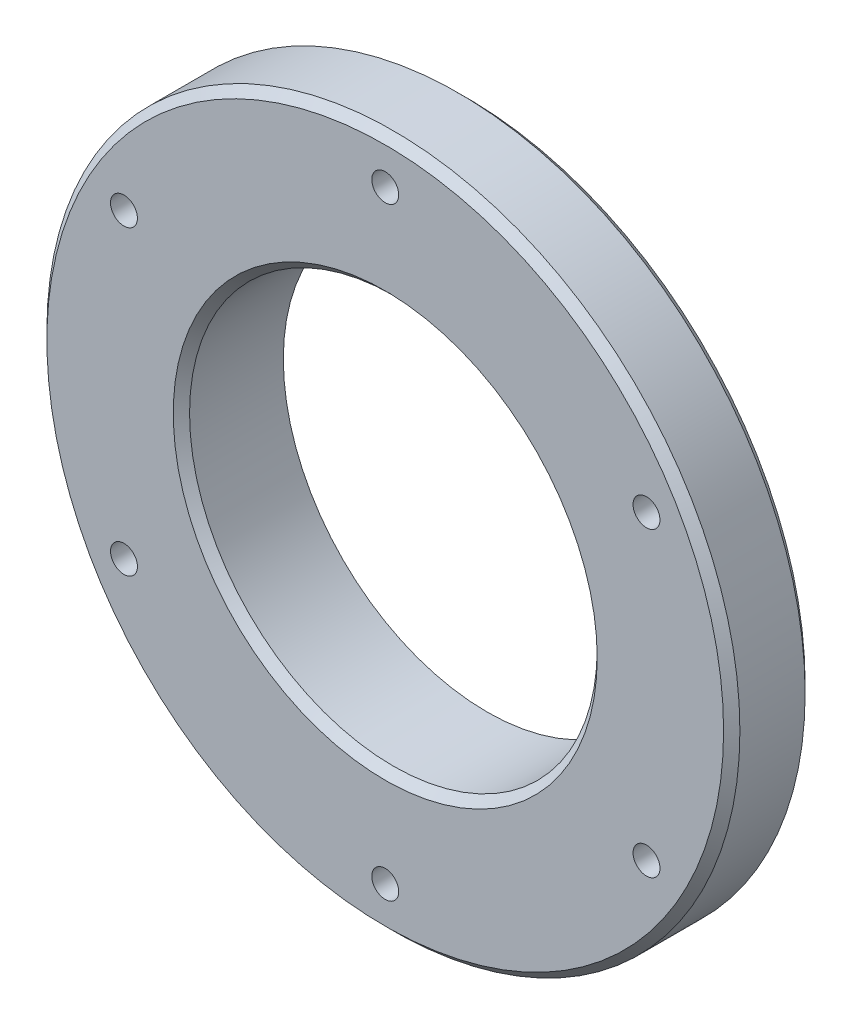
SolidWorks part; units mm, degrees
ref_plane "Front Plane" through (0, 0, 0) normal (0, 0, 1) x (1, 0, 0)
ref_plane "Top Plane" through (0, 0, 0) normal (0, 1, 0) x (1, 0, 0)
ref_plane "Right Plane" through (0, 0, 0) normal (1, 0, 0) x (0, 0, -1)
sketch "Sketch1" plane through (0, 0, 0) normal (0, 0, 1) x (1, 0, 0)
  circle A0 centre (0, 0) radius 42.5
  circle A1 centre (0, 0) radius 25
extrude "Boss-Extrude1" add sketch "Sketch1" along normal blind 10
chamfer "Chamfer1" distance 1 angle 45 3 edges at (42.5, 0, 0) (42.5, 0, 10) (25, 0, 10)
sketch "Sketch2" plane through (0, 0, 10) normal (0, 0, 1) x (1, 0, 0)
  circle A0 centre (0, 37) radius 3.5
  circle A3 centre (32.0434, 18.5009) radius 3.5
  circle A5 centre (32.0444, -18.4991) radius 3.5
  circle A7 centre (0.002, -37) radius 3.5
  circle A9 centre (-32.0414, -18.5009) radius 3.5
  circle A11 centre (-32.0424, 18.4991) radius 3.5
  point P29 (0.001, 0)
  dimension "D1" = 6
hole_wizard "M4x0.7 Tapped Hole1" positions "3DSketch1" profile "Sketch3" tap size "M4x0.7" standard "Ansi Metric"
sketch3d "3DSketch1"
  point P0 (0, 37, 10)
  point P3 (32.0434, 18.5009, 10)
  point P6 (32.0444, -18.4991, 10)
  point P9 (0.002, -37, 10)
  point P12 (-32.0414, -18.5009, 10)
  point P15 (-32.0424, 18.4991, 10)
sketch "Sketch3" plane through (0, 37, 10) normal (1, 0, 0) x (0, -1, 0)
  line L0 (0, 0) -> (0, 6.9914)
  line L1 (0, 6.9914) -> (1.65, 6)
  line L2 (1.65, 6) -> (1.65, 0)
  line L5 (1.65, 0) -> (0, 0)
  line L10 (0, 6.9914) -> (-1.65, 6) construction
  line L11 (0, -6.35) -> (0, 107.95) construction
  dimension "螺纹孔钻头直径" = 3.3
  dimension "螺纹孔钻头深度" = 6
  dimension "导头角度" = 118
cosmetic thread "Cosmetic thread 7" parameters "D1"=6, "D2"=4
cosmetic thread "Cosmetic thread 8" parameters "D1"=6, "D2"=4
cosmetic thread "Cosmetic thread 9" parameters "D1"=6, "D2"=4
cosmetic thread "Cosmetic thread 10" parameters "D1"=6, "D2"=4
cosmetic thread "Cosmetic thread 11" parameters "D1"=6, "D2"=4
cosmetic thread "Cosmetic thread 12" parameters "D1"=6, "D2"=4
sketch "Sketch5" plane through (0, 0, 0) normal (0, 0, -1) x (-1, 0, 0)
  circle A0 centre (0, 0) radius 35
  circle A1 centre (0, 0) radius 25
extrude "Boss-Extrude2" add sketch "Sketch5" along normal blind 2.5
